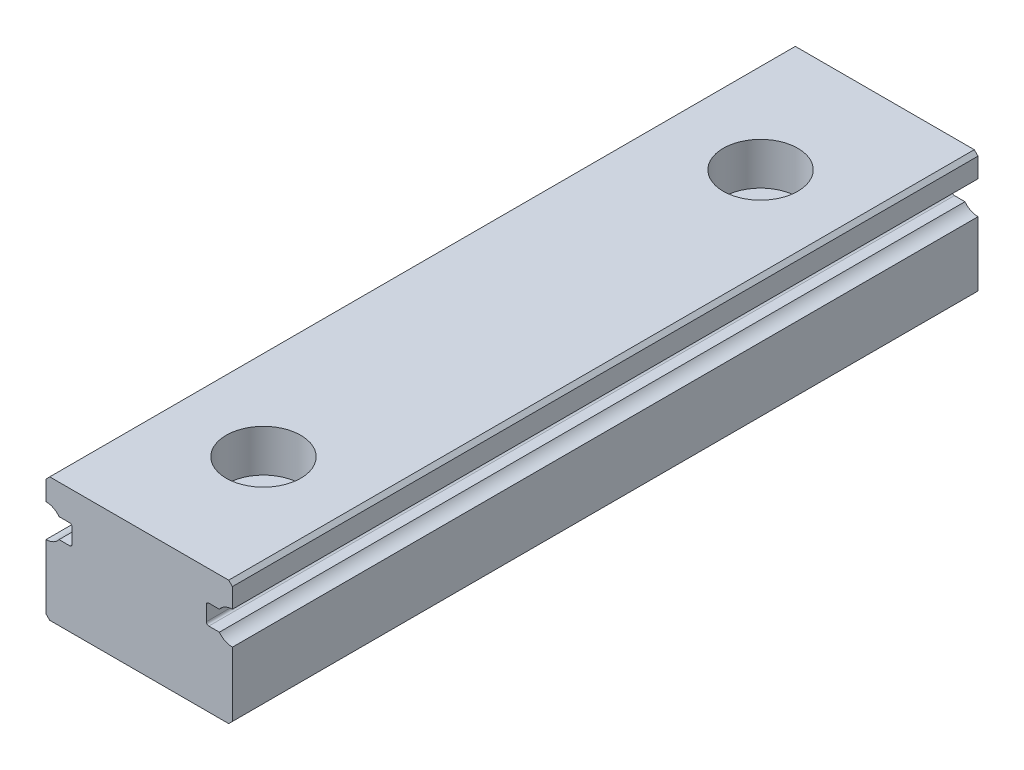
from build123d import *

# Parameters (mm, degrees)
EXTRUDE_1_DEPTH           = 30
HOLE_WIZARD_1_D           = 3.4
HOLE_WIZARD_1_CBORE_D     = 6
HOLE_WIZARD_1_CBORE_DEPTH = 3.4
PATTERN_LINEAR_1_COUNT    = 2
PATTERN_LINEAR_1_PITCH    = 40


with BuildPart() as part:
    # 草图2 → 凸台-拉伸1 (new, symmetric)
    with BuildSketch(Plane.XY):
        with BuildLine():
            Line((7.5, 9.7), (7.2, 10))
            Line((7.2, 10), (-7.2, 10))
            Line((-7.2, 10), (-7.5, 9.7))
            Line((-7.5, 9.7), (-7.5, 8.120037878))
            ThreePointArc((-7.5, 8.120037878), (-6.914137517, 7.982905386), (-6.45, 7.6))
            Line((-6.45, 7.6), (-5.6, 7.6))
            ThreePointArc((-5.6, 7.6), (-5.458578644, 7.541421356), (-5.4, 7.4))
            Line((-5.4, 7.4), (-5.4, 6.2))
            ThreePointArc((-5.4, 6.2), (-5.458578644, 6.058578644), (-5.6, 6))
            Line((-5.6, 6), (-6.45, 6))
            ThreePointArc((-6.45, 6), (-6.914137517, 5.617094614), (-7.5, 5.479962122))
            Line((-7.5, 5.479962122), (-7.5, 0.3))
            Line((-7.5, 0.3), (-7.2, 0))
            Line((-7.2, 0), (7.2, 0))
            Line((7.2, 0), (7.5, 0.3))
            Line((7.5, 0.3), (7.5, 5.479962122))
            ThreePointArc((7.5, 5.479962122), (6.914137517, 5.617094614), (6.45, 6))
            Line((6.45, 6), (5.6, 6))
            ThreePointArc((5.6, 6), (5.458578644, 6.058578644), (5.4, 6.2))
            Line((5.4, 6.2), (5.4, 7.4))
            ThreePointArc((5.4, 7.4), (5.458578644, 7.541421356), (5.6, 7.6))
            Line((5.6, 7.6), (6.45, 7.6))
            ThreePointArc((6.45, 7.6), (6.914137517, 7.982905386), (7.5, 8.120037878))
            Line((7.5, 8.120037878), (7.5, 9.7))
        make_face()
    extrude(amount=EXTRUDE_1_DEPTH, both=True)

    # 打孔尺寸(%根据)内六角圆柱头螺钉的类型1 (through all)
    with Locations(Plane(origin=(0, 10, 20), x_dir=(0, 0, 1), z_dir=(0, 1, 0))):
        with Locations((0, 0)):
            hole_wizard_1 = CounterBoreHole(HOLE_WIZARD_1_D / 2, HOLE_WIZARD_1_CBORE_D / 2, HOLE_WIZARD_1_CBORE_DEPTH)

    # 阵列(线性)1: 打孔尺寸(%根据)内六角圆柱头螺钉的类型1 ×2
    with Locations(*[(0, 0, -i * PATTERN_LINEAR_1_PITCH) for i in range(1, PATTERN_LINEAR_1_COUNT)]):
        add(hole_wizard_1, mode=Mode.SUBTRACT)


solid = part.part
